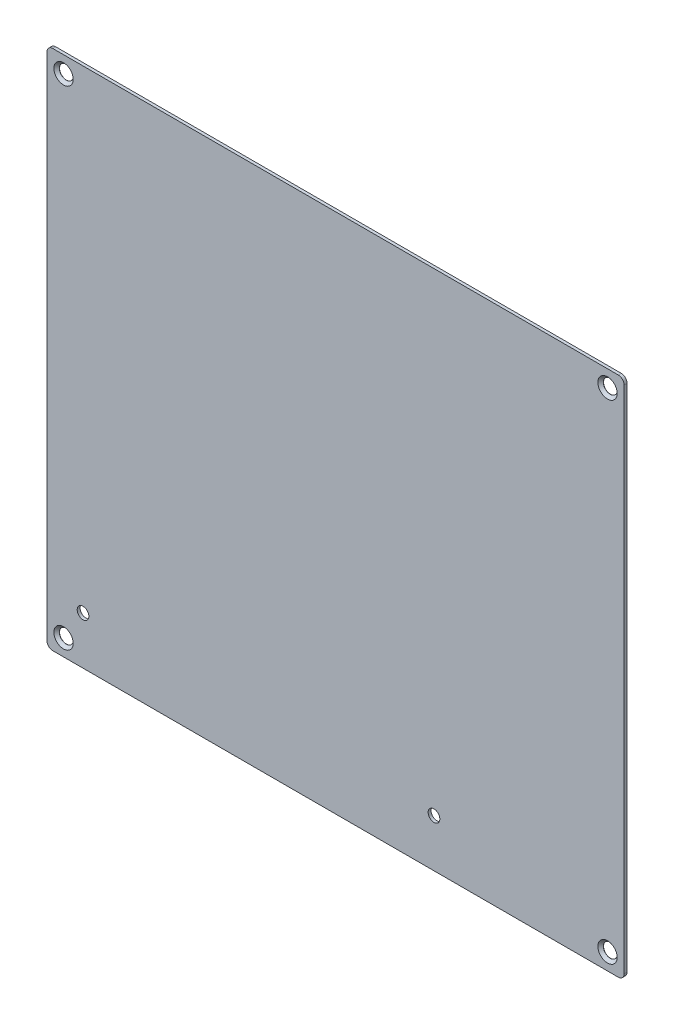
SolidWorks part; units mm, degrees
ref_plane "前视基准面" through (0, 0, 0) normal (0, 0, 1) x (1, 0, 0)
ref_plane "上视基准面" through (0, 0, 0) normal (0, 1, 0) x (1, 0, 0)
ref_plane "右视基准面" through (0, 0, 0) normal (1, 0, 0) x (0, 0, -1)
sketch "草图1" plane through (0, 0, 0) normal (0, 0, 1) x (1, 0, 0)
  line L0 (-89.5, 67) -> (-89.5, 334.5)
  line L1 (-89.5, 334.5) -> (-385.5, 334.5)
  line L2 (-385.5, 334.5) -> (-385.5, 67)
  line L3 (-385.5, 67) -> (-89.5, 67)
extrude "凸台-拉伸1" add sketch "草图1" against normal blind 1.5
hole_wizard "Ø7.1 (7.1) 直径孔2" positions "草图5" profile "草图4" hole size "Ø7.1" standard "ANSI Metric"
sketch "草图5" plane through (0, 0, 0) normal (0, 0, 1) x (1, 0, 0)
  point P0 (-377, 326)
  point P1 (-377, 75.5)
  point P2 (-98, 75.5)
  point P3 (-98, 326)
sketch "草图4" plane through (-377, 326, 0) normal (1, 0, 0) x (0, -1, 0)
  line L0 (0, 0) -> (0, 1.5)
  line L1 (0, 1.5) -> (3.55, 1.5)
  line L2 (3.55, 1.5) -> (3.55, 1.4)
  line L3 (3.55, 1.4) -> (4.95, 0)
  line L5 (4.95, 0) -> (0, 0)
  line L6 (-3.55, 1.4) -> (-4.95, 0) construction
  line L11 (0, -6.35) -> (0, 107.95) construction
  dimension "通孔孔直径" = 7.1
  dimension "通孔孔深度" = 1.5
  dimension "近端锥形沉头孔直径" = 9.9
  dimension "近端锥形沉头孔角度" = 90
fillet "圆角1" radius 3 4 edges at (-89.5, 67, -0.75) (-89.5, 334.5, -0.75) (-385.5, 67, -0.75) (-385.5, 334.5, -0.75)
sketch "草图6" plane through (0, 0, 0) normal (0, 0, 1) x (1, 0, 0)
  line L0 (-382.5, 67) -> (-92.5, 67) construction
  line L1 (-385.5, 331.5) -> (-385.5, 70) construction
  circle A0 centre (-367, 91.5) radius 3
  circle A1 centre (-187, 91.5) radius 3
  dimension "D1" = 6
  dimension "D2" = 24.5
  dimension "D3" = 18.5
  dimension "D4" = 6
  dimension "D5" = 180
extrude "切除-拉伸1" cut sketch "草图6" against normal blind 1.5
